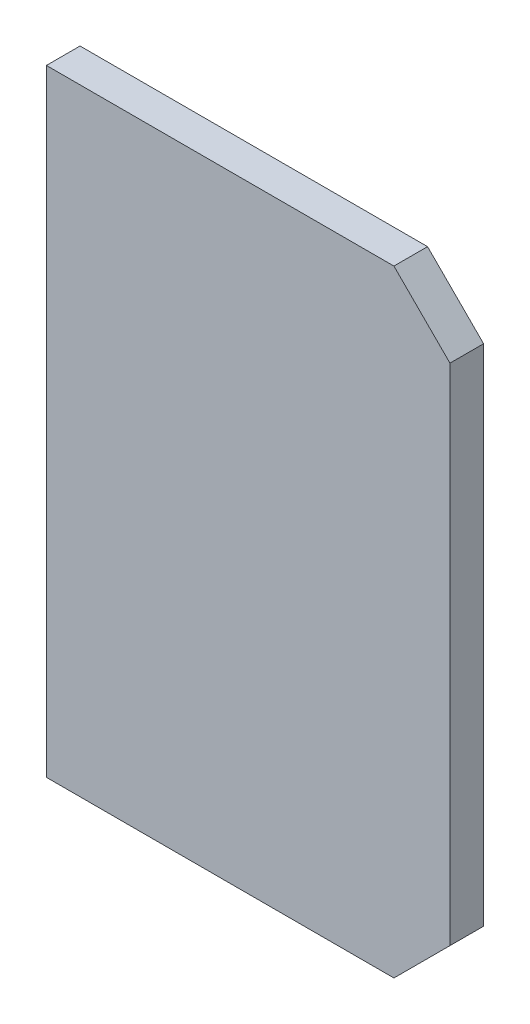
SolidWorks part; units mm, degrees
ref_plane "前视基准面" through (0, 0, 0) normal (0, 0, 1) x (1, 0, 0)
ref_plane "上视基准面" through (0, 0, 0) normal (0, 1, 0) x (1, 0, 0)
ref_plane "右视基准面" through (0, 0, 0) normal (1, 0, 0) x (0, 0, -1)
sketch "草图1" plane through (0, 0, 0) normal (0, 0, 1) x (1, 0, 0)
  line L0 (0, 0) -> (36, 0)
  line L1 (36, 0) -> (36, 55)
  line L2 (36, 55) -> (0, 55)
  line L3 (0, 55) -> (0, 0)
  dimension "D1" = 36
  dimension "D2" = 55
extrude "凸台-拉伸1" add sketch "草图1" along normal blind 3
chamfer "倒角1" distance 5 angle 45 2 edges at (36, 0, 1.5) (36, 55, 1.5)
